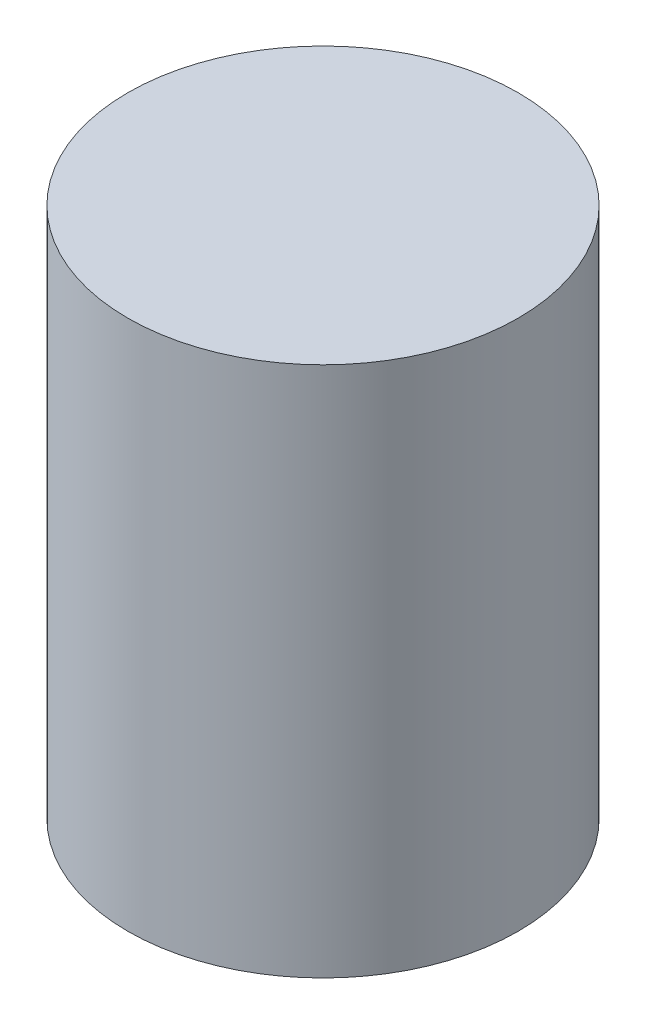
SolidWorks part; units mm, degrees
ref_plane "前视基准面" through (0, 0, 0) normal (0, 0, 1) x (1, 0, 0)
ref_plane "上视基准面" through (0, 0, 0) normal (0, 1, 0) x (1, 0, 0)
ref_plane "右视基准面" through (0, 0, 0) normal (1, 0, 0) x (0, 0, -1)
sketch "草图1" plane through (0, 0, 0) normal (0, 1, 0) x (1, 0, 0)
  circle A0 centre (0, 0) radius 12.5
  dimension "D1" = 25
extrude "凸台-拉伸1" add sketch "草图1" along normal blind 34
